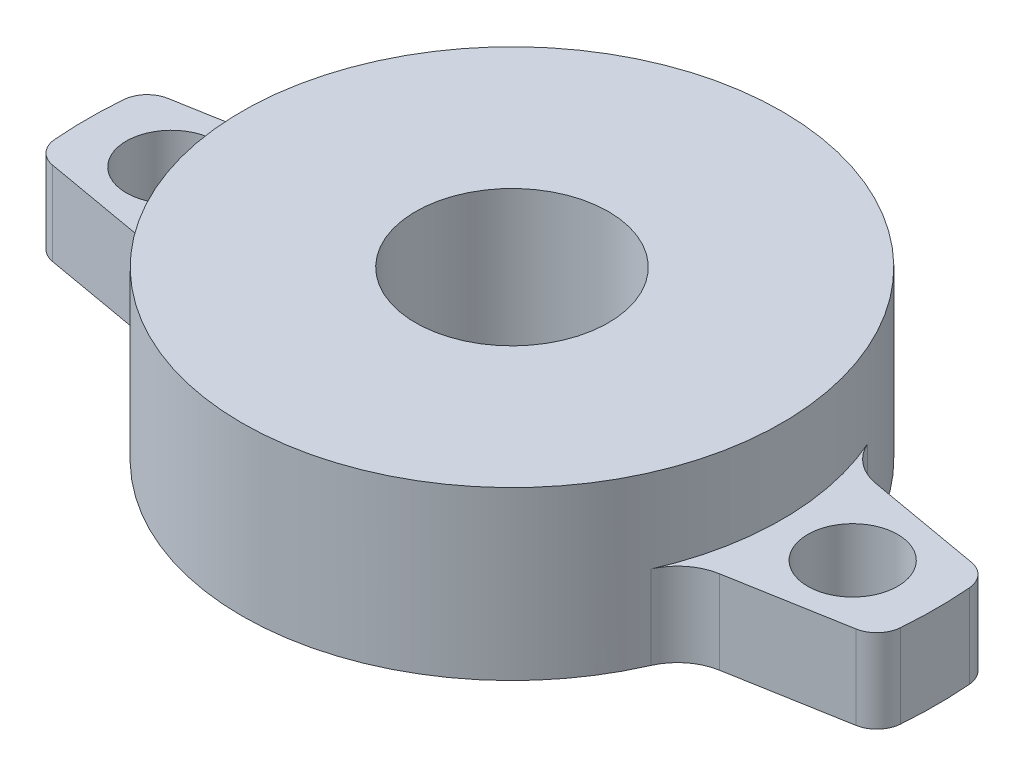
SolidWorks part; units mm, degrees
material "普通碳钢"
ref_plane "前视" through (0, 0, 0) normal (0, 0, 1) x (1, 0, 0)
ref_plane "上视" through (0, 0, 0) normal (0, 1, 0) x (1, 0, 0)
ref_plane "右视" through (0, 0, 0) normal (1, 0, 0) x (0, 0, -1)
sketch "草图1" plane through (0, 0, 0) normal (0, 1, 0) x (1, 0, 0)
  circle A0 centre (0, 0) radius 21
  circle A1 centre (0, 0) radius 7.5
  dimension "D1" = 42
  dimension "D2" = 15
extrude "凸台-拉伸1" add sketch "草图1" along normal blind 13
sketch "草图2" plane through (0, 0, 0) normal (0, -1, 0) x (1, 0, 0)
  line L0 (0, 0) -> (50.6892, 0) construction
  line L1 (0, 0) -> (0, 10) construction
  line L2 (0, 10) -> (32.7279, 4.2292) construction
  line L3 (32.7279, 4.2292) -> (19.976, 6.4777)
  line L4 (32.7279, -4.2292) -> (19.976, -6.4777)
  line L5 (-32.7279, -4.2292) -> (-19.976, -6.4777)
  line L6 (-32.7279, 4.2292) -> (-19.976, 6.4777)
  arc A0 (-32.7279, 4.2292) -> (-32.7279, -4.2292) centre (0, 0) ccw
  circle A1 centre (0, 0) radius 21 construction
  arc A2 (19.976, -6.4777) -> (19.976, 6.4777) centre (0, 0) ccw
  arc A3 (32.7279, -4.2292) -> (32.7279, 4.2292) centre (0, 0) ccw
  arc A4 (-19.976, 6.4777) -> (-19.976, -6.4777) centre (0, 0) ccw
  dimension "D1" = 66
  dimension "D2" = 10
  dimension "D3" = 10
extrude "凸台-拉伸2" add sketch "草图2" against normal blind 6.5
fillet "圆角1" radius 4 4 edges at (-19.976, 3.25, 6.4777) (-19.976, 3.25, -6.4777) (19.976, 3.25, -6.4777) (19.976, 3.25, 6.4777)
fillet "圆角2" radius 2 4 edges at (32.7279, 3.25, 4.2292) (32.7279, 3.25, -4.2292) (-32.7279, 3.25, -4.2292) (-32.7279, 3.25, 4.2292)
sketch "草图3" plane through (0, 6.5, 0) normal (0, 1, 0) x (1, 0, 0)
  circle A0 centre (0, 0) radius 26.5 construction
  circle A1 centre (-26.5, 0) radius 3.5
  circle A2 centre (26.5, 0) radius 3.5
  dimension "D1" = 53
  dimension "D2" = 7
  dimension "D3" = 7
extrude "切除-拉伸1" cut sketch "草图3" against normal blind 6.5
sketch "草图4" plane through (0, 0, 0) normal (0, -1, 0) x (1, 0, 0)
  circle A0 centre (0, 0) radius 18
  dimension "D1" = 36
extrude "切除-拉伸2" cut sketch "草图4" against normal blind 2
